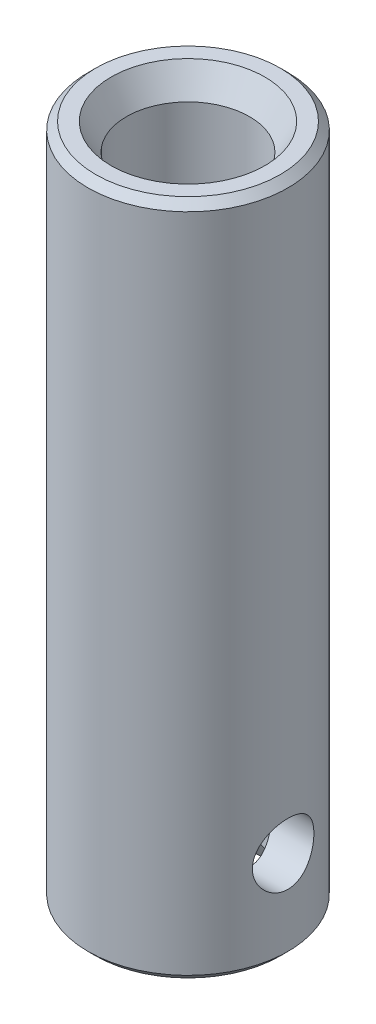
from build123d import *
from OCP.BRepFilletAPI import BRepFilletAPI_MakeChamfer

# Parameters (mm, degrees)
SKETCH_1_R            = 6.5
SKETCH_1_R_2          = 4
EXTRUDE_1_DEPTH       = 44
HOLE_WIZARD_4_0_4_1_D = 4
CHAMFER_1_SIZE        = 0.5
CHAMFER_2_SIZE        = 1
CHAMFER_2_SIZE2       = 1.732050808


with BuildPart() as part:
    # 草图1 → 凸台-拉伸1 (new body)
    with BuildSketch(Plane(origin=(0, 0, 0), x_dir=(1, 0, 0), z_dir=(0, 1, 0))):
        with Locations(Location((0, 0, 0), (0, 0, 270))):
            Circle(SKETCH_1_R)
        with Locations(Location((0, 0, 0), (0, 0, 270))):
            Circle(SKETCH_1_R_2, mode=Mode.SUBTRACT)
    extrude(amount=EXTRUDE_1_DEPTH)

    # Ø4.0 (4) 直径孔1 (through all)
    with Locations(Plane(origin=(6.5, 6, 0), x_dir=(0, 0, 1), z_dir=(1, 0, 0))):
        with Locations((0, 0)):
            Hole(HOLE_WIZARD_4_0_4_1_D / 2)

    # 倒角1
    chamfer_1_edges = [part.edges().sort_by_distance(p)[0] for p in [
        (0, 0, -6.5),
        (0, 44, -6.5),
    ]]
    chamfer(chamfer_1_edges, length=CHAMFER_1_SIZE)

    # 倒角2: one chamfer whose edges measure the first distance from different faces: ONE call of the kernel's chamfer builder (chamfer() names one face for all edges)
    chamfer_2_edges_1 = [part.edges().sort_by_distance(p)[0] for p in [
        (0, 0, -4),
    ]]
    chamfer_2_side_1 = [part.faces().sort_by_distance(p)[0] for p in [
        (0, 0, -5.830294373),
    ]]
    chamfer_2_edges_2 = [part.edges().sort_by_distance(p)[0] for p in [
        (0, 44, -4),
    ]]
    chamfer_2_side_2 = [part.faces().sort_by_distance(p)[0] for p in [
        (0, 44, -5.830294373),
    ]]
    chamfer_2 = BRepFilletAPI_MakeChamfer(part.part.solid().wrapped)
    for e in chamfer_2_edges_1:
        chamfer_2.Add(CHAMFER_2_SIZE, CHAMFER_2_SIZE2, e.wrapped, chamfer_2_side_1[0].wrapped)  # the first distance lies on this face
    for e in chamfer_2_edges_2:
        chamfer_2.Add(CHAMFER_2_SIZE, CHAMFER_2_SIZE2, e.wrapped, chamfer_2_side_2[0].wrapped)  # the first distance lies on this face
    add(Compound.cast(chamfer_2.Shape()), mode=Mode.REPLACE)


solid = part.part
